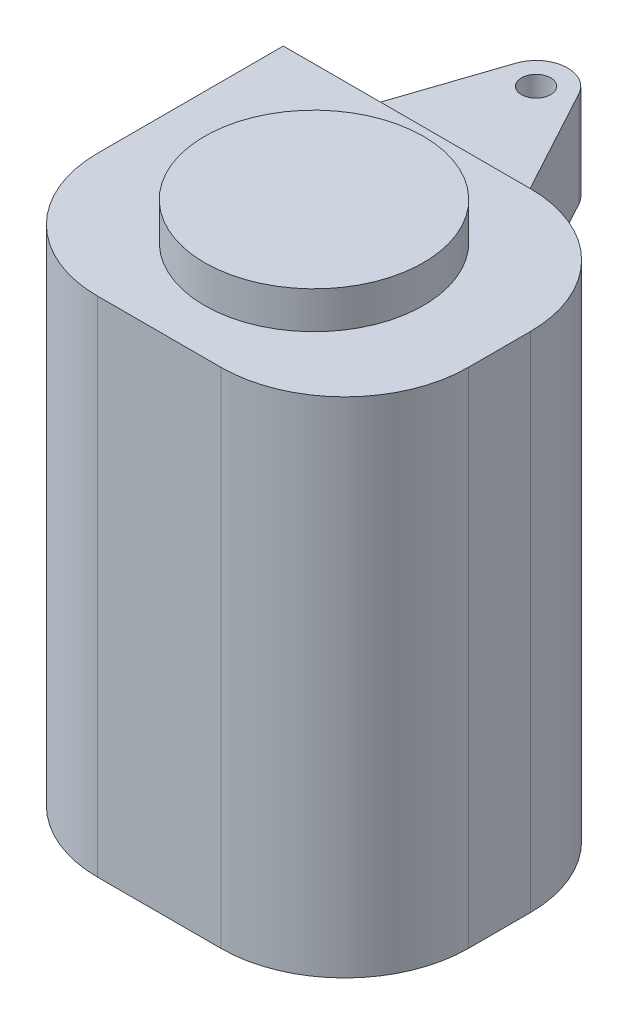
from build123d import *

# Parameters (mm, degrees)
SKETCH1_W           = 29.956211672
SKETCH1_H           = 40.65774509
BOSS_EXTRUDE1_DEPTH = 25
SKETCH2_R           = 1.179493096
BOSS_EXTRUDE2_DEPTH = 17.5
FILLET1_R           = 10
SKETCH3_R           = 8.841541065
BOSS_EXTRUDE3_DEPTH = 3
BOSS_EXTRUDE4_START = 3
SKETCH4_R           = 8.841541065
BOSS_EXTRUDE4_DEPTH = 3
SKETCH5_W           = 18.672217178
SKETCH5_H           = 19.553012946
CUT_EXTRUDE1_DEPTH  = 28


with BuildPart() as part:
    # Sketch1 → Boss-Extrude1 (new body)
    with BuildSketch(Plane.XY):
        with Locations((-25.008704873, 0)):
            Rectangle(SKETCH1_W, SKETCH1_H)
    extrude(amount=BOSS_EXTRUDE1_DEPTH)

    # Sketch2 → Boss-Extrude2 (add, symmetric)
    with BuildSketch(Plane(origin=(0, 0, -4), x_dir=(1, 0, 0), z_dir=(0, -1, 0))):
        with BuildLine():
            Line((-32.216437007, -7.03254357), (-35.914043193, 4))
            Line((-35.914043193, 4), (-21.345745646, 4))
            Line((-21.345745646, 4), (-27.542475863, -7.438106205))
            ThreePointArc((-27.542475863, -7.438106205), (-30.012436117, -8.767867117), (-32.216437007, -7.03254357))
        make_face()
        with Locations(Location((-29.791335202, -6.219759883, 0), (0, 0, 270))):
            Circle(SKETCH2_R, mode=Mode.SUBTRACT)
    extrude(amount=BOSS_EXTRUDE2_DEPTH, both=True)

    # Fillet1
    fillet1_edges = [part.edges().sort_by_distance(p)[0] for p in [
        (-39.986810709, 0, 25),
        (-10.030599037, 0, 25),
        (-10.030599037, 0, 0),
    ]]
    fillet(fillet1_edges, radius=FILLET1_R)

    # Sketch3 → Boss-Extrude3 (add)
    with BuildSketch(Plane(origin=(0, -20.328872545, 0), x_dir=(-1, 0, 0), z_dir=(0, -1, 0))):
        with Locations(Location((25.008704873, -12.5, 0), (0, 0, 90))):
            Circle(SKETCH3_R)
    extrude(amount=BOSS_EXTRUDE3_DEPTH)

    # Sketch4 → Boss-Extrude4 (add)
    with BuildSketch(Plane(origin=(0, 20.328872545, 0), x_dir=(1, 0, 0), z_dir=(0, 1, 0)).offset(BOSS_EXTRUDE4_START)):
        with Locations(Location((-25.008704873, -12.5, 0), (0, 0, 90))):
            Circle(SKETCH4_R)
    extrude(amount=-BOSS_EXTRUDE4_DEPTH)

    # Sketch5 → Cut-Extrude1 (cut)
    with BuildSketch(Plane.ZY.offset(39.986810709)):
        with Locations((-12.777441663, 0)):
            Rectangle(SKETCH5_W, SKETCH5_H)
    extrude(amount=-CUT_EXTRUDE1_DEPTH, mode=Mode.SUBTRACT)


solid = part.part
